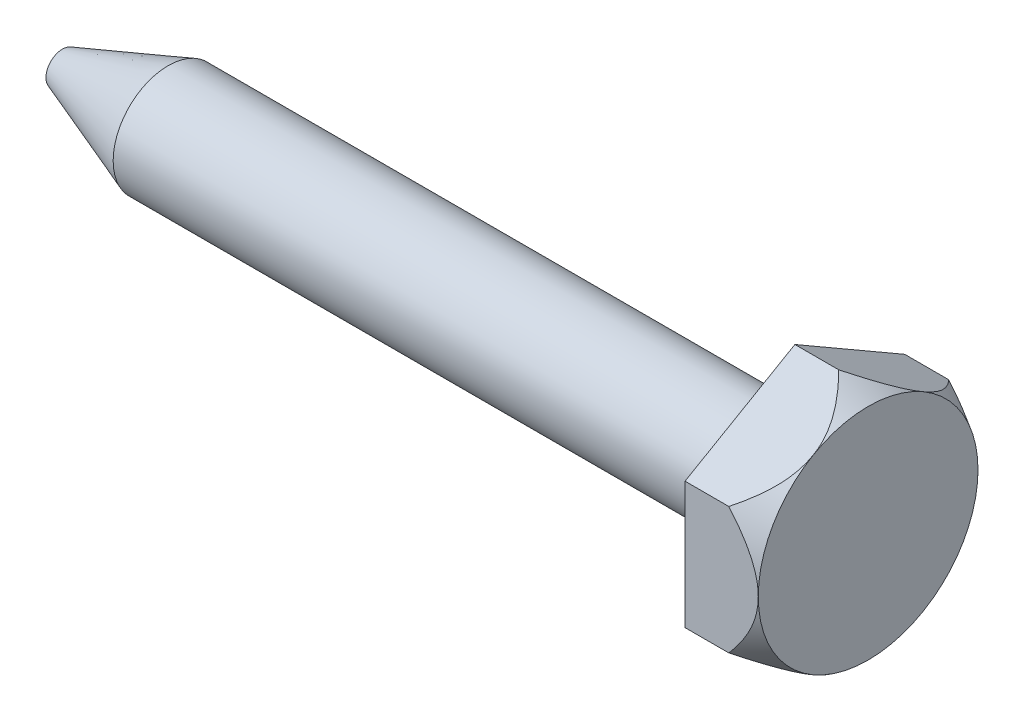
SolidWorks part; units mm, degrees
ref_plane "Front Plane" through (0, 0, 0) normal (0, 0, 1) x (1, 0, 0)
ref_plane "Top Plane" through (0, 0, 0) normal (0, 1, 0) x (1, 0, 0)
ref_plane "Right Plane" through (0, 0, 0) normal (1, 0, 0) x (0, 0, -1)
other "Configuration Table"
sketch "Sketch1" plane through (0, 0, 0) normal (1, 0, 0) x (0, 0, -1)
  line L1 (0, -6.9282) -> (6, -3.4641)
  line L2 (6, -3.4641) -> (6, 3.4641)
  line L3 (6, 3.4641) -> (0, 6.9282)
  line L4 (0, 6.9282) -> (-6, 3.4641)
  line L5 (-6, 3.4641) -> (-6, -3.4641)
  line L6 (-6, -3.4641) -> (0, -6.9282)
  circle A0 centre (0, 0) radius 6 construction
  dimension "D1" = 12
extrude "Boss-Extrude1" add sketch "Sketch1" along normal blind 4
sketch "Sketch2" plane through (4, 0, 0) normal (1, 0, 0) x (0, 0, -1)
  line L0 (6, 3.4641) -> (0, 6.9282) construction
  circle A0 centre (0, 0) radius 6
extrude "Cut-Extrude1" cut sketch "Sketch2" against normal blind 4 draft 30 flip side to cut
sketch "Sketch3" plane through (0, 0, 0) normal (0, 0, 1) x (1, 0, 0)
  line L0 (-29.866, 0) -> (8.7215, 0) construction
  line L1 (0, 3) -> (0, 0)
  line L2 (0, 6.9282) -> (0, 3.4641) construction
  line L3 (0, 0) -> (-40, 0)
  line L4 (-40, 0) -> (-40, 0.9)
  line L5 (-40, 0.9) -> (-34.2303, 3)
  line L6 (-34.2303, 3) -> (0, 3)
  dimension "D1" = 6
  dimension "D2" = 1.8
  dimension "D3" = 20
  dimension "D4" = 40
revolve "Revolve1" add sketch "Sketch3" angle 360 about L0
cosmetic thread "Cosmetic Thread1" parameters "D2"=4.917
